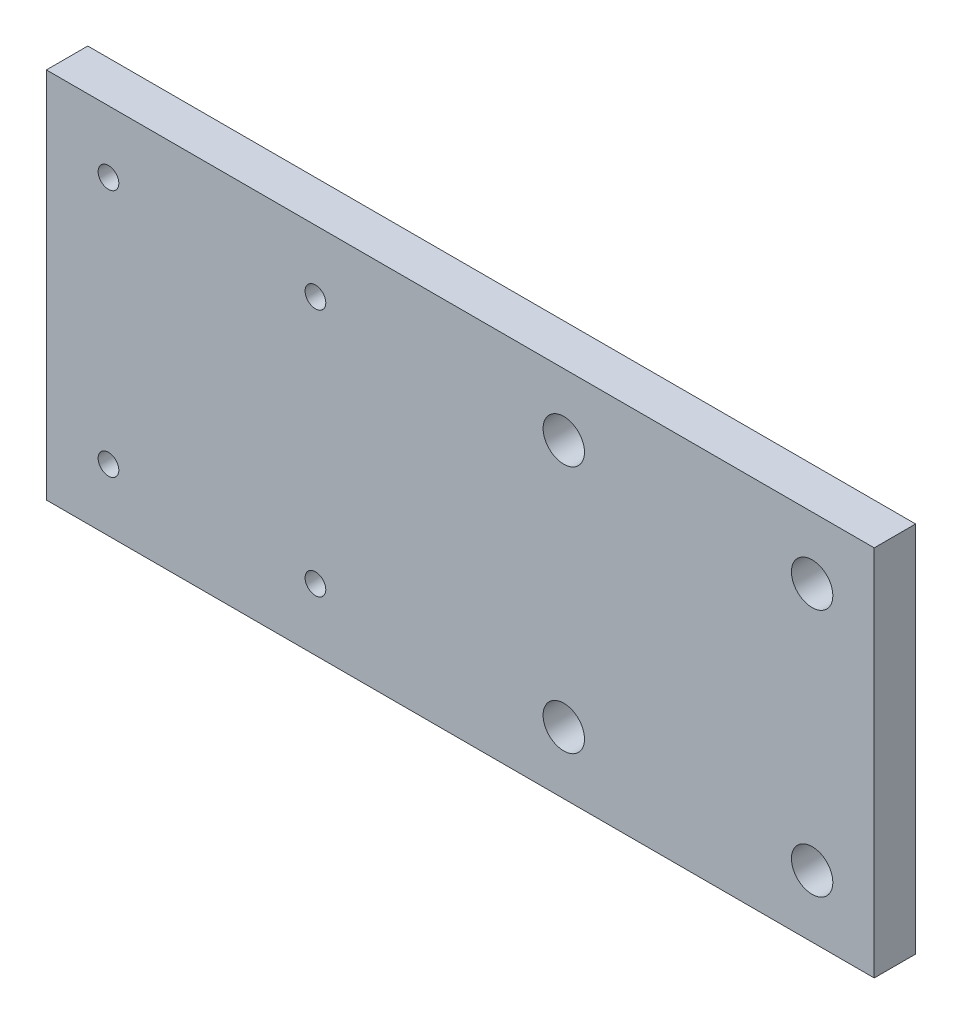
SolidWorks part; units mm, degrees
material "T2"
ref_plane "前视基准面" through (0, 0, 0) normal (0, 0, 1) x (1, 0, 0)
ref_plane "上视基准面" through (0, 0, 0) normal (0, 1, 0) x (1, 0, 0)
ref_plane "右视基准面" through (0, 0, 0) normal (1, 0, 0) x (0, 0, -1)
sketch "草图1" plane through (0, 0, 0) normal (0, 0, 1) x (1, 0, 0)
  line L1 (-100, -45) -> (100, -45)
  line L2 (-100, -45) -> (-100, 45)
  line L3 (-100, 45) -> (100, 45)
  line L4 (100, -45) -> (100, 45)
  line L5 (0, 45) -> (0, -45) construction
  line L6 (-100, 0) -> (100, 0) construction
  point P0 (0, 0)
  dimension "D1" = 90
  dimension "D2" = 200
extrude "凸台-拉伸1" add sketch "草图1" along normal blind 10
sketch "草图2" plane through (0, 0, 10) normal (0, 0, 1) x (1, 0, 0)
  line L0 (-100, -45) -> (100, -45) construction
  line L1 (-100, 45) -> (-10, 45)
  line L2 (-100, 45) -> (-100, -45)
  line L3 (-100, -45) -> (-10, -45)
  line L4 (-10, 45) -> (-10, -45)
  dimension "D1" = 90
extrude "切除-拉伸1" [suppressed] cut sketch "草图2" against normal blind 10
sketch "草图3" plane through (0, 0, 0) normal (0, 0, -1) x (-1, 0, 0)
  line L0 (-100, 45) -> (100, 45) construction
  line L1 (-100, -45) -> (-10, -45)
  line L2 (-100, -45) -> (-100, 45)
  line L3 (-100, 45) -> (-10, 45)
  line L4 (-10, -45) -> (-10, 45)
  dimension "D1" = 90
extrude "切除-拉伸2" [suppressed] cut sketch "草图3" against normal blind 10
hole_wizard "M6 螺纹孔1" positions "草图4" profile "草图5" tap size "M6" standard "GB" end condition through all
sketch "草图4" plane through (0, 0, 0) normal (0, 0, -1) x (-1, 0, 0)
  line L0 (100, 0) -> (-68.3884, 0) construction
  line L1 (100, 45) -> (100, -45) construction
  line L4 (85, 30) -> (35, 30) construction
  line L5 (85, 30) -> (85, -30) construction
  line L6 (85, -30) -> (35, -30) construction
  line L7 (35, 30) -> (35, -30) construction
  line L8 (60, -30) -> (60, 30) construction
  line L9 (85, 0) -> (35, 0) construction
  point P9 (35, -30)
  point P203 (85, -30)
  point P204 (35, 30)
  point P216 (85, 30)
  point P224 (0, 0)
  point P225 (-68.3884, 0)
  dimension "D1" = 50
  dimension "D2" = 60
  dimension "D3" = 15
sketch "草图5" plane through (-85, 30, 0) normal (1, 0, 0) x (0, 1, 0)
  line L0 (0, 0) -> (0, 10)
  line L1 (0, 10) -> (2.5, 10)
  line L2 (2.5, 10) -> (2.5, 0)
  line L5 (2.5, 0) -> (0, 0)
  line L11 (0, -6.35) -> (0, 107.95) construction
  dimension "通孔螺纹孔钻头直径" = 5
  dimension "通孔螺纹孔钻头深度" = 10
cosmetic thread "孔螺蚊线1"
cosmetic thread "孔螺蚊线2"
cosmetic thread "孔螺蚊线3"
cosmetic thread "孔螺蚊线4"
hole_wizard "M8 间隙孔1" positions "草图6" profile "草图7" hole size "M8" standard "GB"
sketch "草图6" plane through (0, 0, 10) normal (0, 0, 1) x (1, 0, 0)
  line L0 (0, 0) -> (100, 0) construction
  line L1 (100, -45) -> (100, 45) construction
  line L3 (25, -30) -> (85, -30) construction
  line L4 (25, -30) -> (25, 30) construction
  line L5 (25, 30) -> (85, 30) construction
  line L6 (85, -30) -> (85, 30) construction
  line L7 (55, 30) -> (55, -30) construction
  line L8 (25, 0) -> (85, 0) construction
  point P8 (85, 30)
  point P165 (25, -30)
  point P166 (25, 30)
  point P167 (85, -30)
  dimension "D1" = 60
  dimension "D2" = 60
  dimension "D3" = 15
sketch "草图7" plane through (85, -30, 10) normal (1, 0, 0) x (0, -1, 0)
  line L0 (0, 0) -> (0, 33.0043)
  line L1 (0, 33.0043) -> (5, 30)
  line L2 (5, 30) -> (5, 0)
  line L5 (5, 0) -> (0, 0)
  line L10 (0, 33.0043) -> (-5, 30) construction
  line L11 (0, -6.35) -> (0, 107.95) construction
  dimension "孔直径" = 10
  dimension "孔深度" = 30
  dimension "导头角度" = 118
